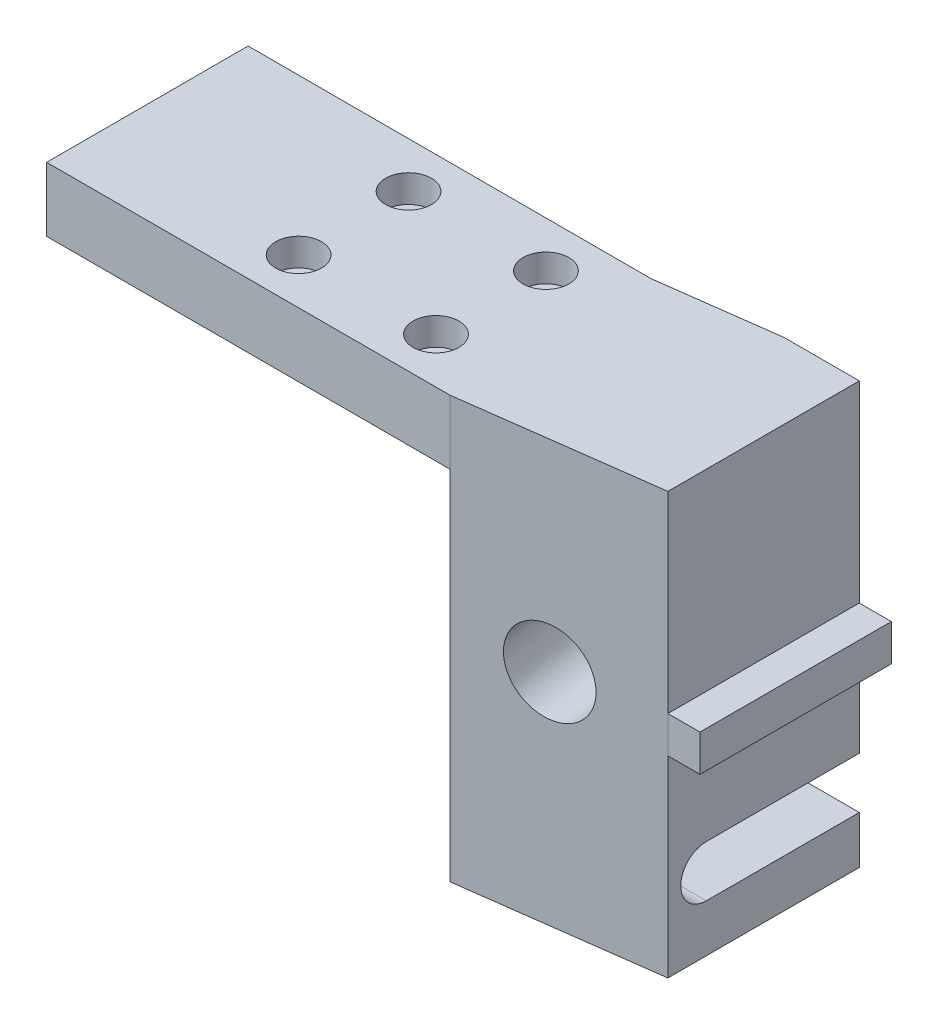
SolidWorks part; units mm, degrees
material "6061 合金"
ref_plane "前视基准面" through (0, 0, 0) normal (0, 0, 1) x (1, 0, 0)
ref_plane "上视基准面" through (0, 0, 0) normal (0, 1, 0) x (1, 0, 0)
ref_plane "右视基准面" through (0, 0, 0) normal (1, 0, 0) x (0, 0, -1)
sketch "草图1" plane through (0, 0, 0) normal (0, 0, 1) x (1, 0, 0)
  line L1 (-47.875, 22.6875) -> (20.635, 22.6875)
  line L2 (-47.875, 22.6875) -> (-47.875, -23.3125)
  line L3 (-47.875, -23.3125) -> (20.635, -23.3125)
  line L4 (20.635, 22.6875) -> (20.635, -23.3125)
  dimension "D1" = 46
  dimension "D2" = 68.51
extrude "凸台-拉伸1" add sketch "草图1" along normal blind 23.69
sketch "草图3" plane through (20.635, 0, 0) normal (1, 0, 0) x (0, 0, -1)
  line L3 (0, -23.3125) -> (0, 22.6875) construction
  line L4 (0, -18.1125) -> (-16.69, -18.1125)
  line L6 (0, -12.5125) -> (-16.69, -12.5125)
  line L8 (-23.69, -23.3125) -> (0, -23.3125) construction
  line L9 (0, -12.5125) -> (0, -18.1125)
  arc A1 (-16.69, -12.5125) -> (-16.69, -18.1125) centre (-16.69, -15.3125) ccw
  dimension "D1" = 5.2
  dimension "D2" = 5.6
  dimension "D3" = 16.69
extrude "切除-拉伸1" cut sketch "草图3" against normal up to next
sketch "草图4" plane through (0, 22.6875, 0) normal (0, 1, 0) x (1, 0, 0)
  line L0 (20.635, -23.69) -> (20.635, -20.89)
  line L1 (20.635, -23.69) -> (20.635, 0) construction
  line L2 (20.635, -20.89) -> (17.135, -20.89)
  line L3 (17.135, -20.89) -> (-3.865, -23.69)
  line L4 (20.635, -23.69) -> (-47.875, -23.69) construction
  line L5 (-3.865, -23.69) -> (20.635, -23.69)
  line L6 (-47.875, 0) -> (-47.875, -1.7)
  line L7 (-47.875, -23.69) -> (-47.875, 0) construction
  line L8 (-47.875, -1.7) -> (-3.875, -1.7)
  line L9 (-3.875, -1.7) -> (8.925, 0)
  line L10 (20.635, 0) -> (-47.875, 0) construction
  line L11 (8.925, 0) -> (-47.875, 0)
  dimension "D1" = 24.5
  dimension "D2" = 2.8
  dimension "D3" = 3.5
  dimension "D4" = 56.8
  dimension "D5" = 44
  dimension "D6" = 1.7
extrude "切除-拉伸2" cut sketch "草图4" against normal up to next
sketch "草图5" plane through (0, 0, 23.69) normal (0, 0, 1) x (1, 0, 0)
  line L0 (20.635, -2.3125) -> (17.135, -2.3125)
  line L1 (20.635, -23.3125) -> (17.135, -23.3125)
  line L2 (20.635, -23.3125) -> (20.635, -2.3125)
  line L3 (20.635, 22.6875) -> (17.135, 22.6875)
  line L5 (17.135, -23.3125) -> (17.135, 22.6875) construction
  line L6 (17.135, -2.3125) -> (17.135, -23.3125)
  line L7 (20.635, 1.6875) -> (17.135, 1.6875)
  line L8 (17.135, 1.6875) -> (17.135, 22.6875)
  line L9 (-3.865, -23.3125) -> (-3.865, 15.6875)
  line L10 (-3.865, -23.3125) -> (-3.865, 22.6875) construction
  line L12 (20.635, 1.6875) -> (20.635, 22.6875)
  line L14 (-3.865, 15.6875) -> (-47.875, 15.6875)
  line L15 (-47.875, 22.6875) -> (-47.875, -23.3125) construction
  line L16 (-47.875, 15.6875) -> (-47.875, -23.3125)
  line L17 (-47.875, -23.3125) -> (-3.865, -23.3125)
  dimension "D1" = 21
  dimension "D2" = 21
  dimension "D3" = 39
extrude "切除-拉伸3" cut sketch "草图5" against normal up to next
sketch "草图6" plane through (0.1547, 0, 1.1648) normal (-0.1317, 0, -0.9913) x (-0.9913, 0, 0.1317)
  line L0 (-8.8473, -12.5125) -> (4.055, -12.5125) construction
  line L1 (4.055, 15.6875) -> (4.055, -12.5125) construction
  circle A0 centre (-2.755, 0.6875) radius 4.5
  dimension "D1" = 9
  dimension "D2" = 13.2
  dimension "D3" = 6.81
extrude "切除-拉伸4" cut sketch "草图6" against normal up to next
sketch "草图9" plane through (0, 22.6875, 0) normal (0, 1, 0) x (1, 0, 0)
  line L0 (-47.875, -23.69) -> (-47.875, -1.7) construction
  line L1 (-3.865, -23.69) -> (-47.875, -23.69) construction
  circle A0 centre (-25.375, -6.69) radius 1.45
  circle A1 centre (-25.375, -18.69) radius 1.45
  circle A2 centre (-10.375, -18.69) radius 1.45
  circle A3 centre (-10.375, -6.69) radius 1.45
  dimension "D1" = 2.9
  dimension "D4" = 22.5
  dimension "D5" = 5
  dimension "D2" = 2
  dimension "D3" = 2
extrude "切除-拉伸5" cut sketch "草图9" against normal up to next
sketch "草图11" plane through (0, 22.6875, 0) normal (0, 1, 0) x (1, 0, 0)
  circle A0 centre (-25.375, -6.69) radius 2.5
  circle A1 centre (-10.375, -6.69) radius 2.5
  circle A2 centre (-25.375, -18.69) radius 2.5
  circle A3 centre (-10.375, -18.69) radius 2.5
  dimension "D1" = 5
  dimension "D2" = 2
  dimension "D3" = 2
extrude "切除-拉伸6" cut sketch "草图11" against normal blind 3
